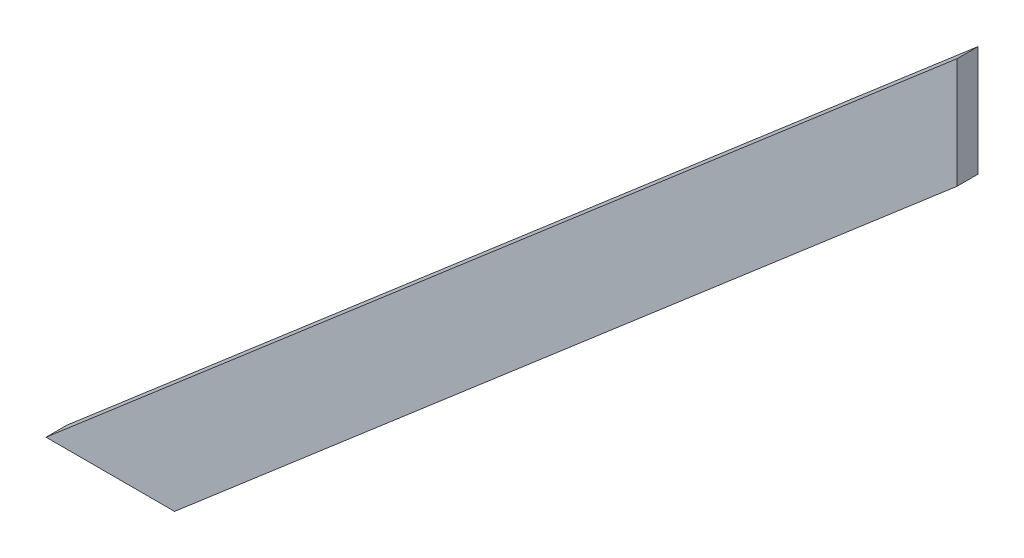
SolidWorks part; units mm, degrees
ref_plane "Front Plane" through (0, 0, 0) normal (0, 0, 1) x (1, 0, 0)
ref_plane "Top Plane" through (0, 0, 0) normal (0, 1, 0) x (1, 0, 0)
ref_plane "Right Plane" through (0, 0, 0) normal (1, 0, 0) x (0, 0, -1)
other "Configuration Table"
sketch "Sketch1" plane through (0, 0, 0) normal (0, 0, 1) x (1, 0, 0)
  line L8 (-1213.3835, 12946.4072) -> (-906.6203, 12946.4072)
  line L9 (-906.6203, 12946.4072) -> (960.4822, 14551.813)
  line L10 (960.4822, 14551.813) -> (960.4822, 14815.5796)
  line L11 (960.4822, 14815.5796) -> (-1213.3835, 12946.4072)
extrude "Boss-Extrude1" add sketch "Sketch1" along normal blind 50
